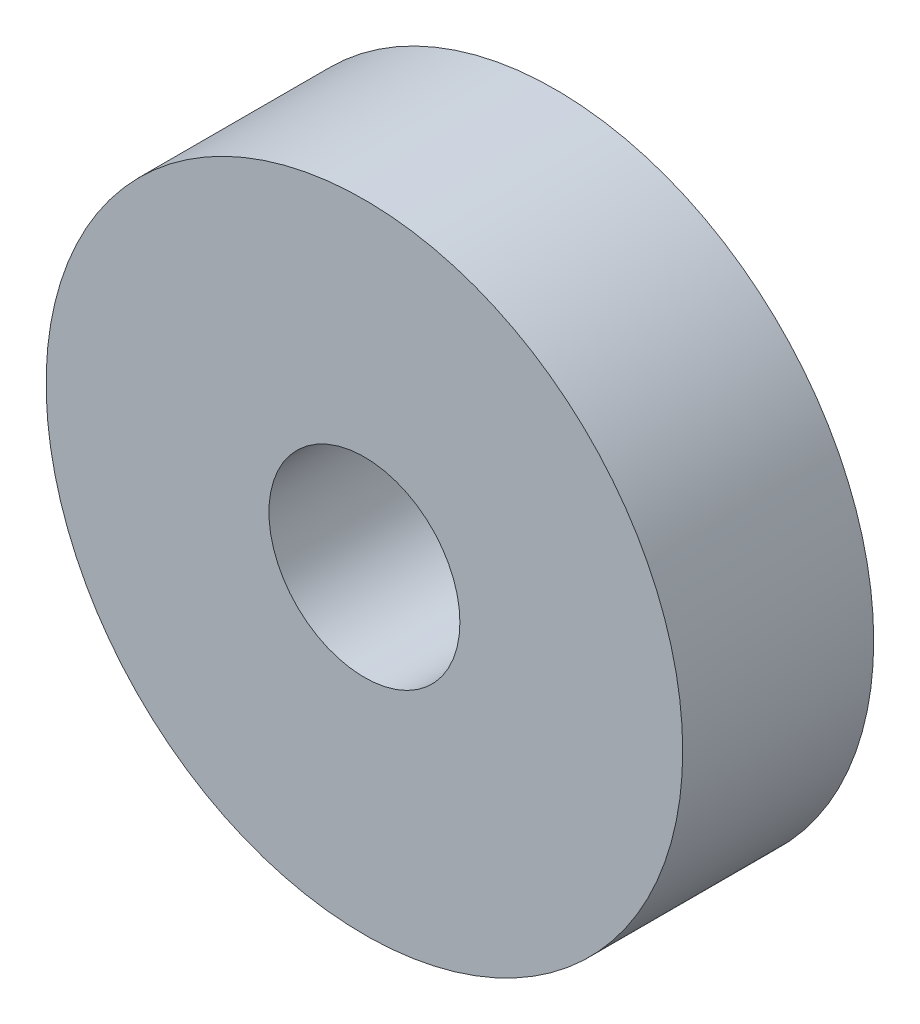
from build123d import *

# Parameters (mm, degrees)
SKETCH1_R           = 10
SKETCH1_R_2         = 3
BOSS_EXTRUDE1_DEPTH = 6


with BuildPart() as part:
    # Sketch1 → Boss-Extrude1 (new body)
    with BuildSketch(Plane.XY):
        Circle(SKETCH1_R)
        Circle(SKETCH1_R_2, mode=Mode.SUBTRACT)
    extrude(amount=BOSS_EXTRUDE1_DEPTH)


solid = part.part
